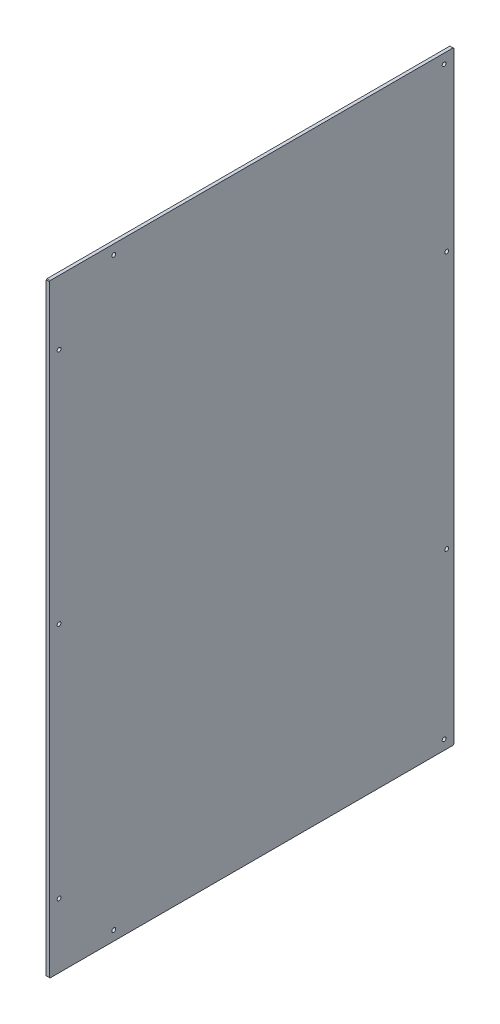
from build123d import *

# Parameters (mm, degrees)
SKETCH_1_W          = 628
SKETCH_1_H          = 938
EXTRUDE_1_DEPTH     = 5
CHAMFER_1_SIZE      = 1
SKETCH_2_R          = 3
CUT_EXTRUDE_1_DEPTH = 565.430686621


with BuildPart() as part:
    # 草图1 → 凸台-拉伸1 (new body)
    with BuildSketch(Plane(origin=(0, 0, 0), x_dir=(0, 0, -1), z_dir=(1, 0, 0))):
        Rectangle(SKETCH_1_W, SKETCH_1_H)
    extrude(amount=EXTRUDE_1_DEPTH)

    # 倒角1
    chamfer_1_edges = [part.edges().sort_by_distance(p)[0] for p in [
        (2.5, 469, 314),
        (2.5, 469, -314),
        (2.5, -469, -314),
        (2.5, -469, 314),
    ]]
    chamfer(chamfer_1_edges, length=CHAMFER_1_SIZE)

    # 草图2 → 切除-拉伸1 (cut, through all)
    with BuildSketch(Plane.ZY):
        with Locations((-299, 454)):
            Circle(SKETCH_2_R)
        with Locations(Location((-299, -454, 0), (0, 0, 180))):
            Circle(SKETCH_2_R)
        with Locations((214, 454)):
            Circle(SKETCH_2_R)
        with Locations((299, 369)):
            Circle(SKETCH_2_R)
        with Locations((299, -369)):
            Circle(SKETCH_2_R)
        with Locations((214, -454)):
            Circle(SKETCH_2_R)
        with Locations((299, 0)):
            Circle(SKETCH_2_R)
        with Locations((-303, 200)):
            Circle(SKETCH_2_R)
        with Locations((-303, -200)):
            Circle(SKETCH_2_R)
    extrude(amount=-CUT_EXTRUDE_1_DEPTH, mode=Mode.SUBTRACT)


solid = part.part
